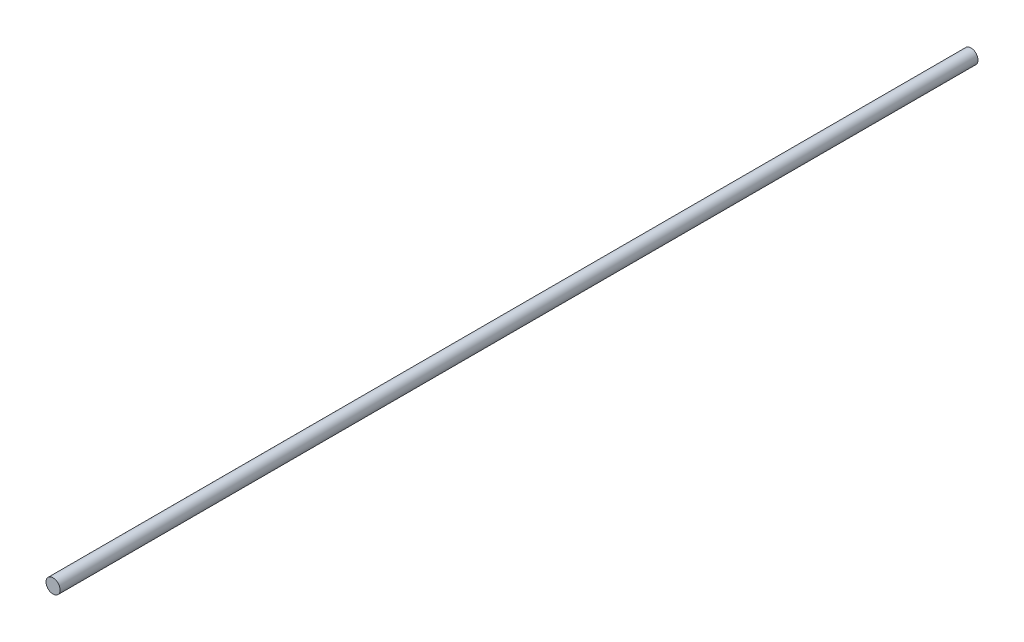
from build123d import *

# Parameters (mm, degrees)
SKETCH_1_R      = 10
EXTRUDE_1_DEPTH = 650


with BuildPart() as part:
    # 草图1 → 凸台-拉伸1 (new, symmetric)
    with BuildSketch(Plane.XY):
        Circle(SKETCH_1_R)
    extrude(amount=EXTRUDE_1_DEPTH, both=True)


solid = part.part
